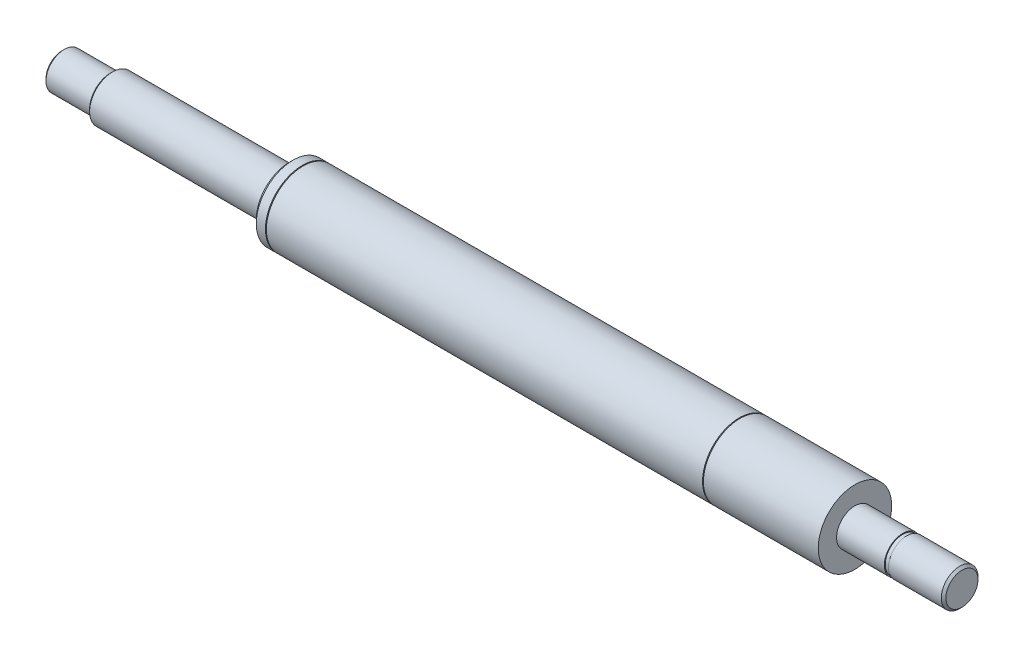
from build123d import *

# Parameters (mm, degrees)
SKETCH2_W     = 0.2
SKETCH2_H     = 1.6
SKETCH2_W_2   = 0.9
SKETCH2_H_2   = 0.2
CHAMFER1_SIZE = 0.5
CHAMFER2_SIZE = 0.8


with BuildPart() as part:
    # Sketch1 → Revolve1 (revolve)
    with BuildSketch(Plane(origin=(0, 0, 0), x_dir=(1, 0, 0), z_dir=(0, 1, 0))):
        Polygon((0, 0), (0, -4), (10.5, -4), (10.5, -5), (49.5, -5), (49.5, -8), (172.7, -8), (172.7, -4), (196, -4), (196, 0), align=None)
    revolve(axis=Axis((-12.256689328, 0, 0), (1, 0, 0)))

    # Sketch2 → Cut-Revolve1 (revolve, cut)
    with BuildSketch(Plane(origin=(0, 0, 0), x_dir=(1, 0, 0), z_dir=(0, 1, 0))):
        with Locations((52.4, -7.2)):
            Rectangle(SKETCH2_W, SKETCH2_H)
        with Locations((147.6, -7.2)):
            Rectangle(SKETCH2_W, SKETCH2_H)
        with Locations((183.55, -3.9)):
            Rectangle(SKETCH2_W_2, SKETCH2_H_2)
    revolve(axis=Axis((-6.355227553, 0, 0), (1, 0, 0)), mode=Mode.SUBTRACT)

    # Chamfer1
    chamfer1_edges = [part.edges().sort_by_distance(p)[0] for p in [
        (0, 0, -4),
        (196, 0, -4),
        (10.5, 0, -5),
    ]]
    chamfer(chamfer1_edges, length=CHAMFER1_SIZE)

    # Chamfer2
    chamfer2_edges = [part.edges().sort_by_distance(p)[0] for p in [
        (49.5, 0, -8),
    ]]
    chamfer(chamfer2_edges, length=CHAMFER2_SIZE)


solid = part.part
